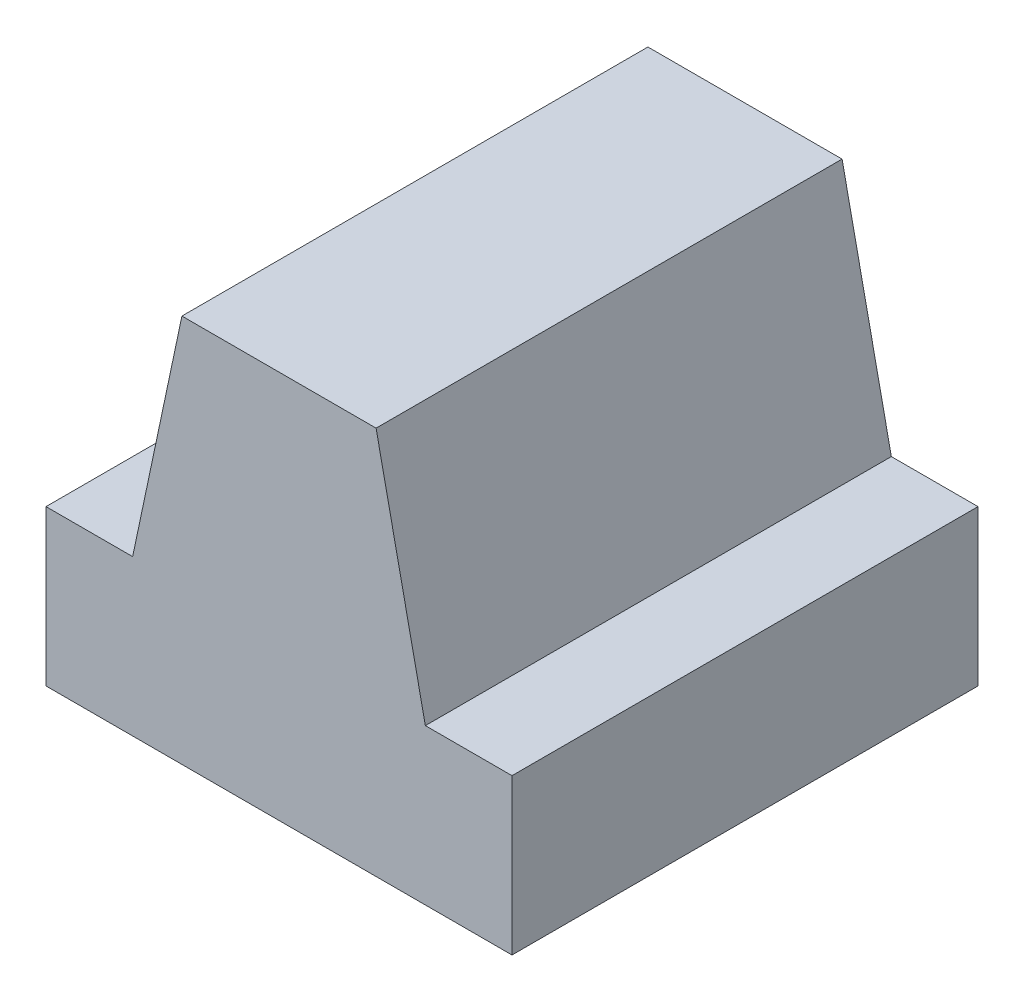
from build123d import *

# Parameters (mm, degrees)
BOSS_EXTRUDE1_DEPTH = 6


with BuildPart() as part:
    # Sketch1 → Boss-Extrude1 (new body)
    with BuildSketch(Plane.XY):
        Polygon((-3, 0), (0, 0), (0, 5), (-1.25, 5), (-1.884373414, 2), (-3, 2), align=None)
        Polygon((0, 5), (0, 0), (3, 0), (3, 2), (1.884373414, 2), (1.25, 5), align=None)
    extrude(amount=BOSS_EXTRUDE1_DEPTH)


solid = part.part
